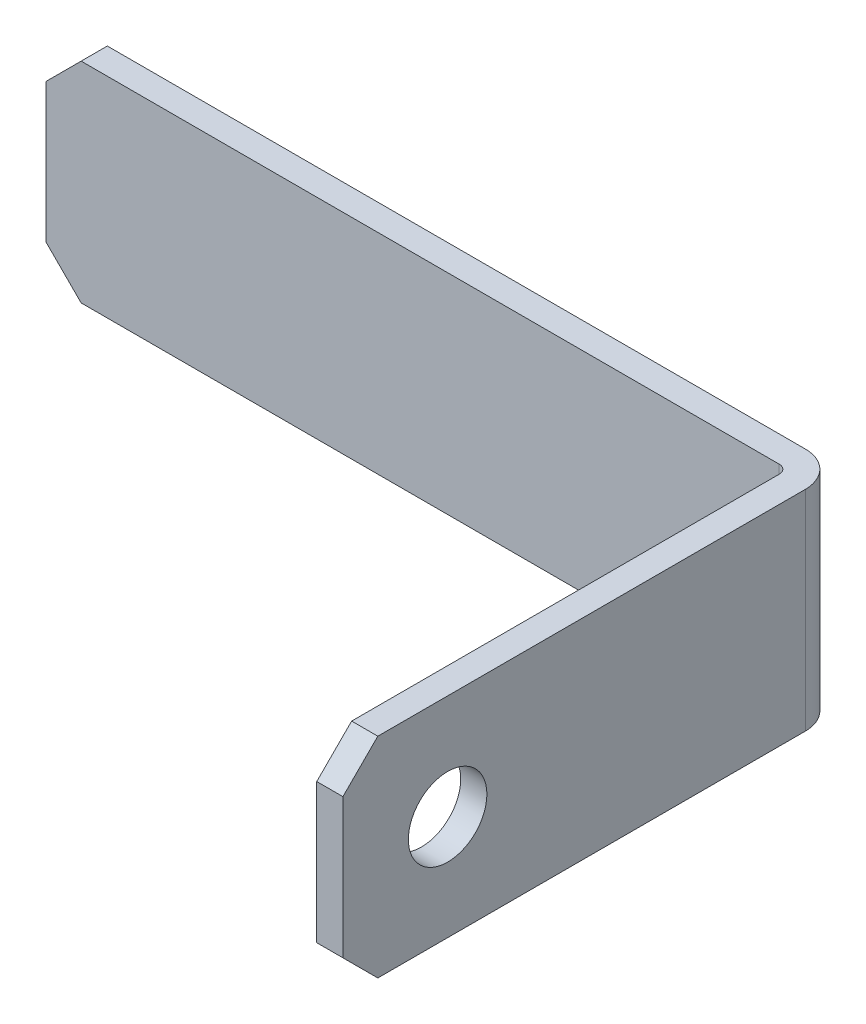
from build123d import *

# Parameters (mm, degrees)
BOSS_EXTRUDE1_DEPTH = 12
SKETCH2_R           = 2.25
CUT_EXTRUDE1_DEPTH  = 54.779642989
CHAMFER1_SIZE       = 2
FILLET1_R           = 2
FILLET2_R           = 0.5


with BuildPart() as part:
    # Sketch1 → Boss-Extrude1 (new body)
    with BuildSketch(Plane(origin=(0, 0, 0), x_dir=(1, 0, 0), z_dir=(0, 1, 0))):
        Polygon((0, 0), (-1.5, 0), (-1.5, 27), (-44, 27), (-44, 28.5), (0, 28.5), align=None)
    extrude(amount=BOSS_EXTRUDE1_DEPTH)

    # Sketch2 → Cut-Extrude1 (cut, through all)
    with BuildSketch(Plane(origin=(0, 0, 0), x_dir=(0, 0, -1), z_dir=(1, 0, 0))):
        with Locations((6, 6)):
            Circle(SKETCH2_R)
    extrude(amount=-CUT_EXTRUDE1_DEPTH, mode=Mode.SUBTRACT)

    # Chamfer1
    chamfer1_edges = [part.edges().sort_by_distance(p)[0] for p in [
        (-44, 12, -27.75),
        (-0.75, 12, 0),
        (-0.75, 0, 0),
        (-44, 0, -27.75),
    ]]
    chamfer(chamfer1_edges, length=CHAMFER1_SIZE)

    # Fillet1
    fillet1_edges = [part.edges().sort_by_distance(p)[0] for p in [
        (0, 6, -28.5),
    ]]
    fillet(fillet1_edges, radius=FILLET1_R)

    # Fillet2
    fillet2_edges = [part.edges().sort_by_distance(p)[0] for p in [
        (-1.5, 6, -27),
    ]]
    fillet(fillet2_edges, radius=FILLET2_R)


solid = part.part
